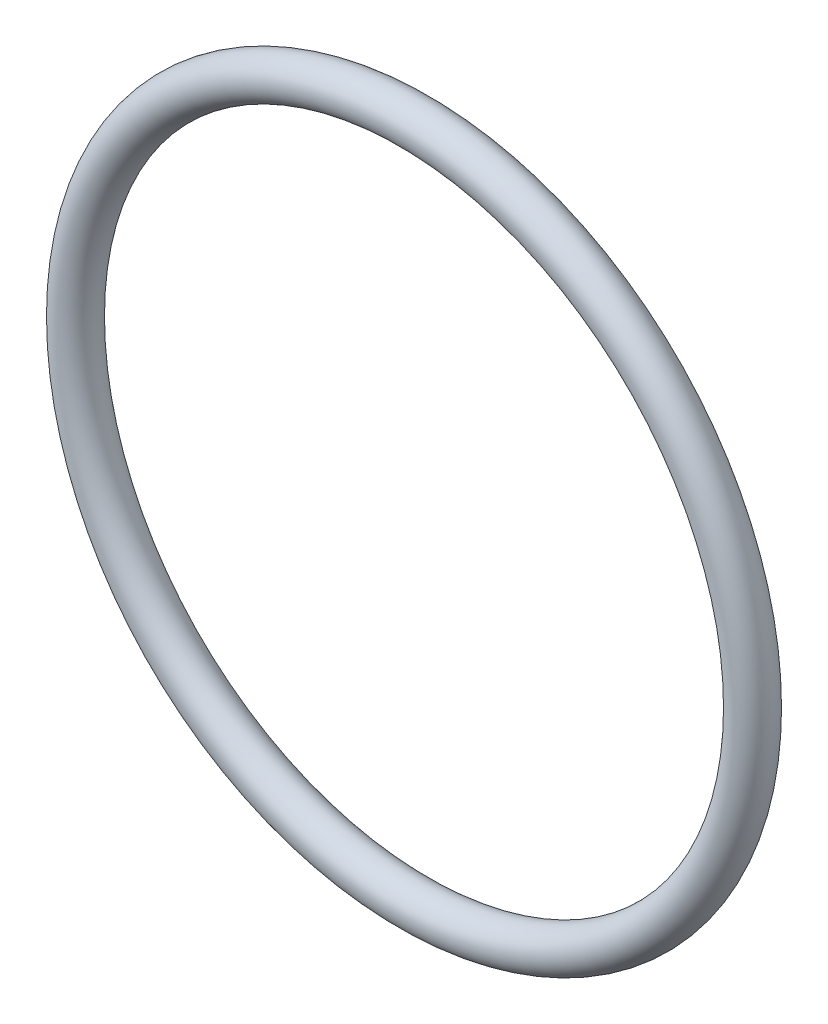
from build123d import *

# Parameters (mm, degrees)
SKETCH2_R = 0.5


with BuildPart() as part:
    # Sweep1: sweep along a path in Sketch1
    with BuildLine(Plane.XY) as sweep1_path:
        CenterArc((0, 0), 8.25, 0, 360)
    # Sketch2 → Sweep1 (sweep)
    with BuildSketch(Plane(origin=(0, 0, 0), x_dir=(1, 0, 0), z_dir=(0, 1, 0))):
        with Locations((-8.25, 0)):
            Circle(SKETCH2_R)
    sweep(path=sweep1_path.line)


solid = part.part
